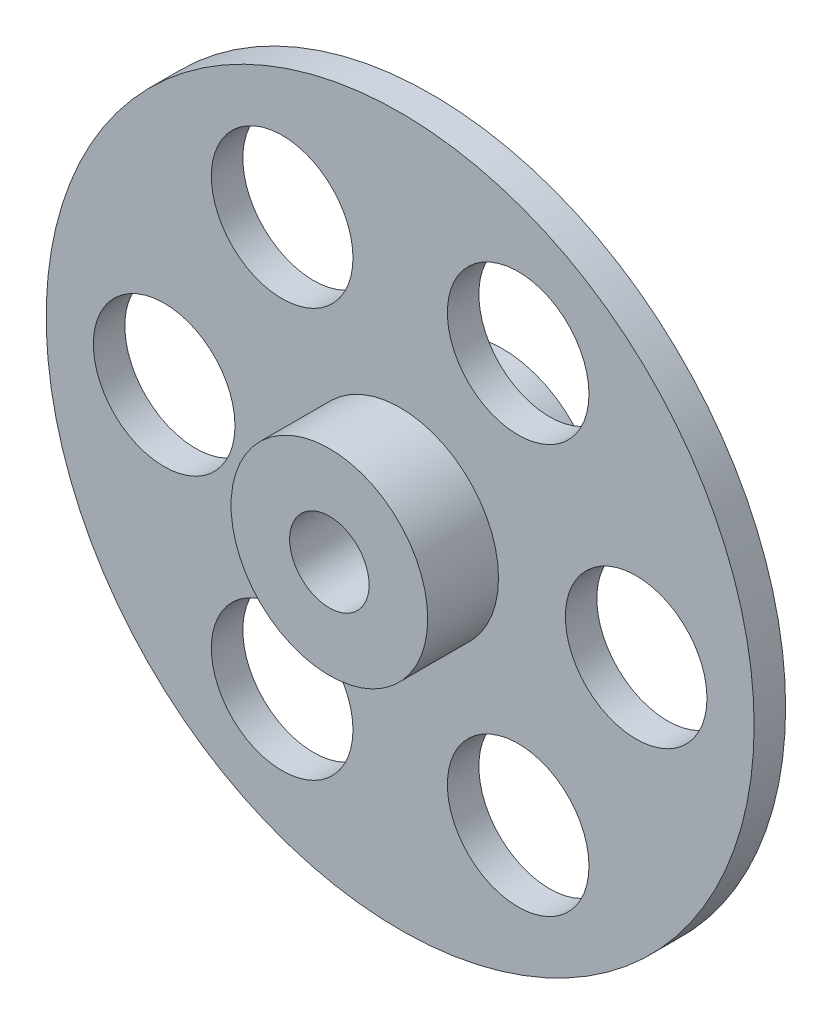
from build123d import *

# Parameters (mm, degrees)
SKETCH_1_R          = 90
SKETCH_1_R_2        = 10.1
EXTRUDE_1_DEPTH     = 4
SKETCH_2_R          = 25
SKETCH_2_R_2        = 10.1
EXTRUDE_2_DEPTH     = 22
SKETCH_3_R          = 18
CUT_EXTRUDE_1_DEPTH = 30


with BuildPart() as part:
    # 草图1 → 凸台-拉伸1 (new, symmetric)
    with BuildSketch(Plane.XY):
        Circle(SKETCH_1_R)
        Circle(SKETCH_1_R_2, mode=Mode.SUBTRACT)
    extrude(amount=EXTRUDE_1_DEPTH, both=True)

    # 草图2 → 凸台-拉伸2 (add, symmetric)
    with BuildSketch(Plane.XY):
        Circle(SKETCH_2_R)
        Circle(SKETCH_2_R_2, mode=Mode.SUBTRACT)
    extrude(amount=EXTRUDE_2_DEPTH, both=True)

    # 草图3 → 切除-拉伸1 (cut, symmetric)
    with BuildSketch(Plane.XY):
        with Locations((60, 0)):
            Circle(SKETCH_3_R)
        with Locations((30, 51.961524227)):
            Circle(SKETCH_3_R)
        with Locations((-30, 51.961524227)):
            Circle(SKETCH_3_R)
        with Locations((-60, 0)):
            Circle(SKETCH_3_R)
        with Locations((-30, -51.961524227)):
            Circle(SKETCH_3_R)
        with Locations((30, -51.961524227)):
            Circle(SKETCH_3_R)
    extrude(amount=CUT_EXTRUDE_1_DEPTH, both=True, mode=Mode.SUBTRACT)


solid = part.part
